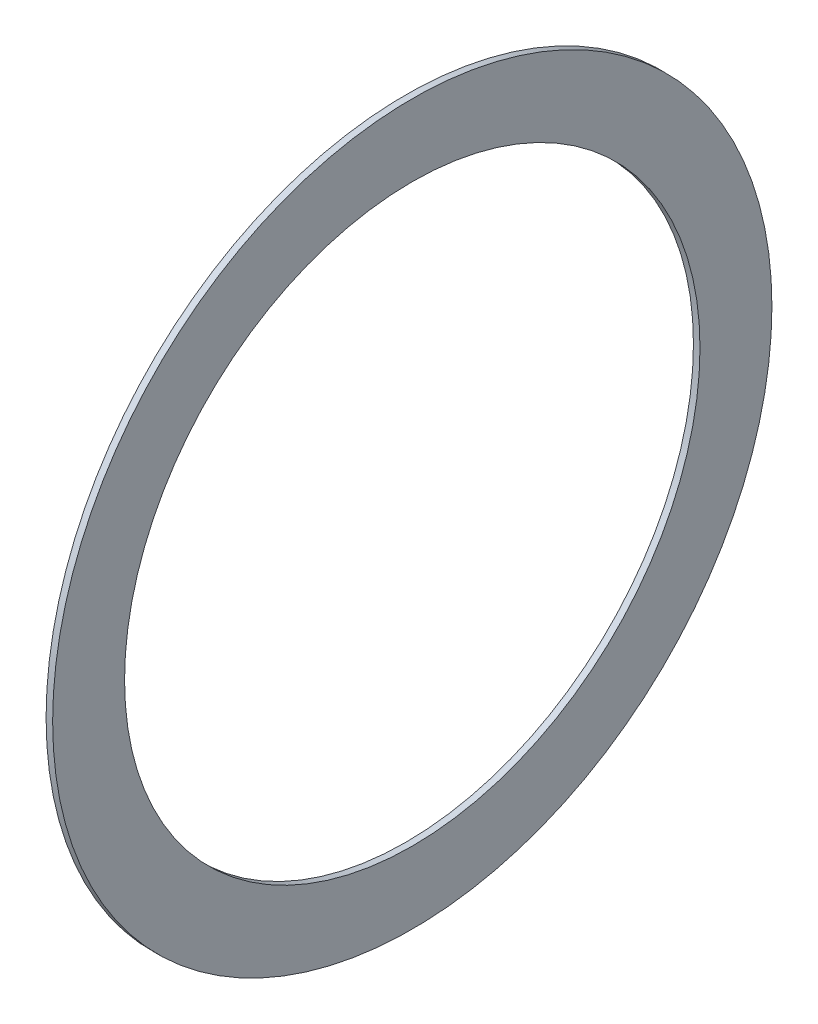
from build123d import *

# Parameters (mm, degrees)
SKETCH_1_R      = 22.5
SKETCH_1_R_2    = 18
EXTRUDE_1_DEPTH = 0.41


with BuildPart() as part:
    # 草图1 → 凸台-拉伸1 (new body)
    with BuildSketch(Plane(origin=(0, 0, 0), x_dir=(0, 0, -1), z_dir=(1, 0, 0))):
        Circle(SKETCH_1_R)
        Circle(SKETCH_1_R_2, mode=Mode.SUBTRACT)
    extrude(amount=EXTRUDE_1_DEPTH)


solid = part.part
